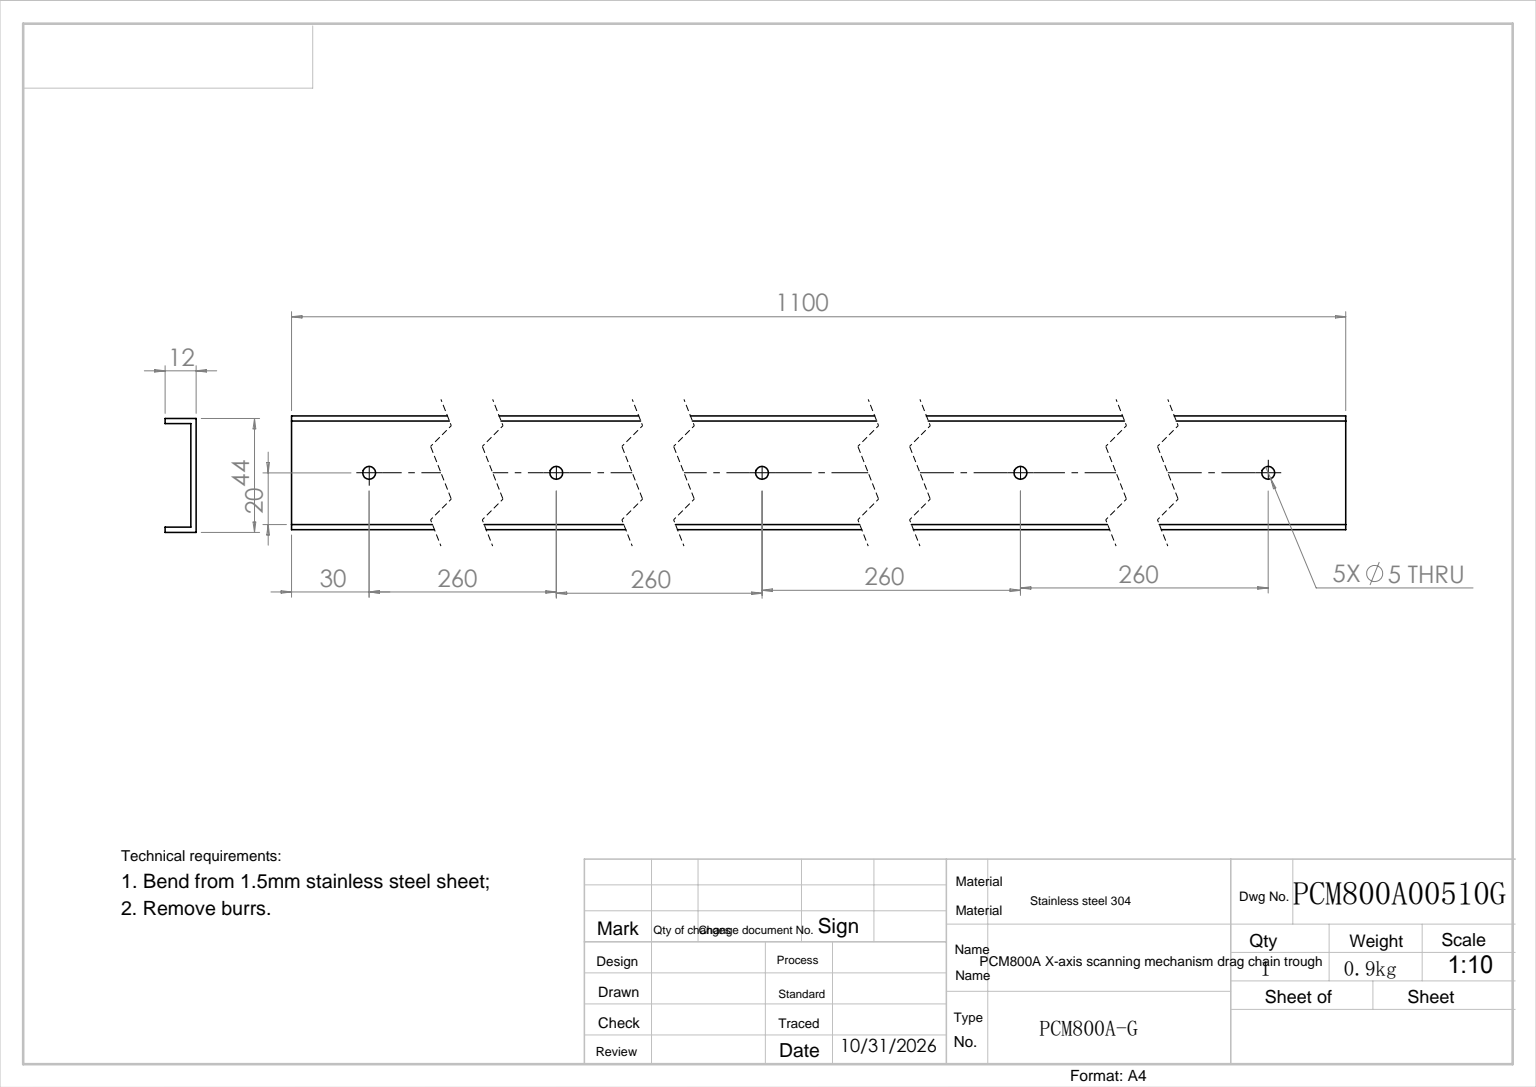
SolidWorks part; units mm, degrees
ref_plane "前视基准面" through (0, 0, 0) normal (0, 0, 1) x (1, 0, 0)
ref_plane "上视基准面" through (0, 0, 0) normal (0, 1, 0) x (1, 0, 0)
ref_plane "右视基准面" through (0, 0, 0) normal (1, 0, 0) x (0, 0, -1)
sketch "草图1" plane through (0, 0, 0) normal (0, 0, 1) x (1, 0, 0)
  line L0 (0, 0) -> (0, -10)
  line L1 (0, -10) -> (40, -10)
  line L2 (-2, 0) -> (-2, -12)
  line L3 (-2, -12) -> (42, -12)
  line L4 (-2, 0) -> (0, 0)
  line L5 (-2, -12) -> (40, -12) construction
  line L6 (42, -12) -> (42, 0)
  line L7 (42, 0) -> (40, 0)
  line L8 (40, 0) -> (40, -10)
  dimension "D1" = 10
  dimension "D2" = 40
  dimension "D3" = 2
  dimension "D4" = 2
extrude "凸台-拉伸1" add sketch "草图1" along normal blind 1100
sketch "草图2" plane through (0, -10, 0) normal (0, 1, 0) x (1, 0, 0)
  line L1 (40, 0) -> (0, 0) construction
  line L2 (40, -1100) -> (40, 0) construction
  circle A0 centre (20, -30) radius 2.5
  dimension "D1" = 5
  dimension "D2" = 20
  dimension "D3" = 30
extrude "切除-拉伸1" cut sketch "草图2" against normal through all
pattern_linear "阵列(线性)1" count 5 spacing 260 along (0, 0, 1) of "切除-拉伸1"
